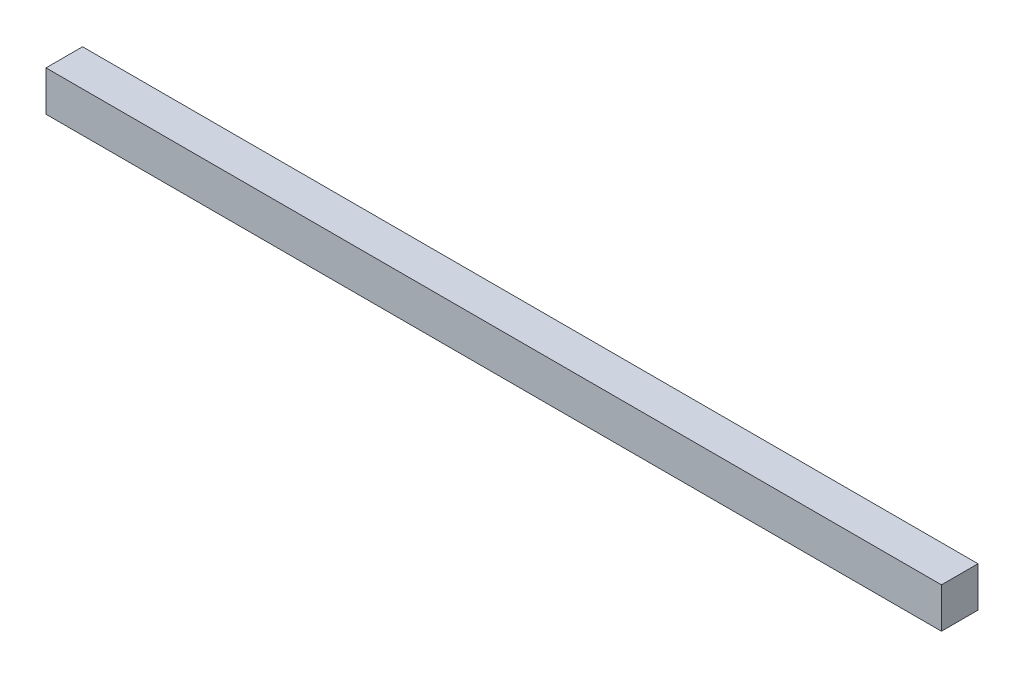
SolidWorks part; units mm, degrees
material "Q235B"
ref_plane "Front Plane" through (0, 0, 0) normal (0, 0, 1) x (1, 0, 0)
ref_plane "Top Plane" through (0, 0, 0) normal (0, 1, 0) x (1, 0, 0)
ref_plane "Right Plane" through (0, 0, 0) normal (1, 0, 0) x (0, 0, -1)
sketch "Sketch1" plane through (0, 0, 0) normal (0, 0, 1) x (1, 0, 0)
  line L1 (0, 0) -> (490, 0)
  line L2 (0, 0) -> (0, 22)
  line L3 (0, 22) -> (490, 22)
  line L4 (490, 0) -> (490, 22)
  dimension "D1" = 490
  dimension "D2" = 22
extrude "Boss-Extrude1" add sketch "Sketch1" along normal blind 20
